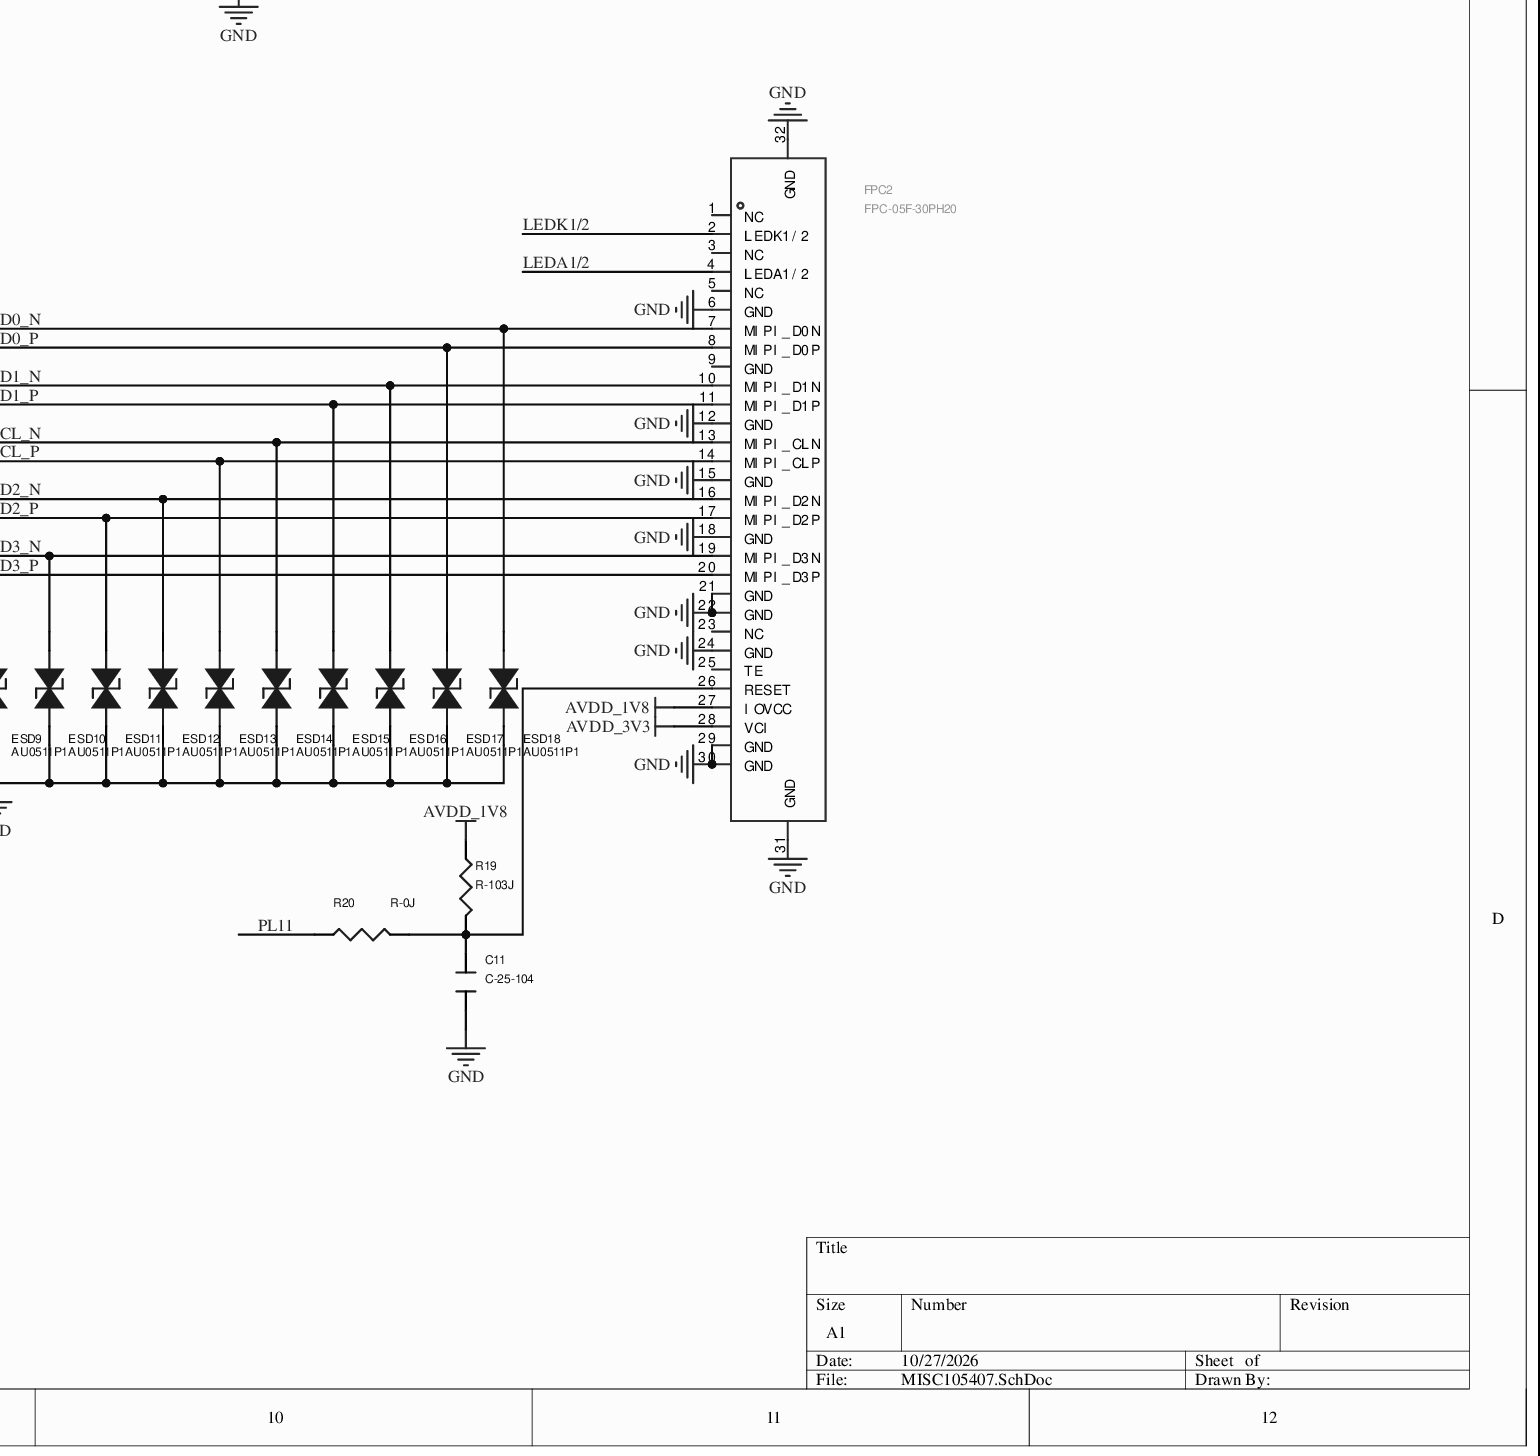
[diagram p0: MISC105407.SchDoc, bottom column 4 of 4]
# Altium project MISC105407.PrjPcb (part 3 of 3)

## Sheet MISC105407.SchDoc
size A1; SheetNumber: 1; SheetTotal: 1

### Parts
C1  C-16-225(±10%)  [C0402]
C2  C-50-104(±10%)  [C0402]
C3  C-25-104  [C0402]
C4  C-25-104  [C0402]
C5  C-25-104  [C0402]
C6  C-25-106  [C0603]
C7  C-25-104  [C0402]
C8  C-25-106  [C0603]
C9  C-25-104  [C0402]
C10  C-25-104  [C0402]
C11  C-25-104  [C0402]
C12  C-50-105  [C0402]
C13  C-25-106  [C0603]
C14  C-50-330  [C0402]
C15  C-50-104  [C0402]
C16  C-16-106(±10%)  [C0603]
C17  C-16-106(±10%)  [C0603]
C18  C-50-472(±10%)  [C0402]
C19  C-16-106(±10%)  [C0603]
C20  C-50-220(±10%)  [C0402]
C21  C-16-106(±10%)  [C0603]
C22  C-16-106(±10%)  [C0603]
C23  C-16-106(±10%)  [C0603]
C24  C-50-101  [C0402]
C25  C-50-106  [C0603]
C26  C-50-104  [C0402]
C27  C-50-330  [C0402]
D1  1N5819  [SOD323]
D2  AU0511P1  [ESD0402A]
D3  AU0511P1  [ESD0402A]
D4  1N5819  [SOD323]
D5  AU0511P1  [ESD0402A]
D6  AU0511P1  [ESD0402A]
D7  AU0511P1  [ESD0402A]
D8  AU0511P1  [ESD0402A]
D9  AU0511P1  [ESD0402A]
D10  AU0511P1  [ESD0402A]
D11  AU0511P1  [ESD0402A]
D12  AU0511P1  [ESD0402A]
D13  AU0511P1  [ESD0402A]
D14  AU0511P1  [ESD0402A]
D15  SS34F_C18199199  [SMAF_L3.5-W2.6-LS4.7-RD-1]
D16  SS34F_C18199199  [SMAF_L3.5-W2.6-LS4.7-RD-1]
D17  AU0511P1  [ESD0402A]
D18  AU0511P1  [ESD0402A]
D19  AU0511P1  [ESD0402A]
D20  AU0511P1  [ESD0402A]
D21  AU0511P1  [ESD0402A]
D22  AU0511P1  [ESD0402A]
ESD1  AU0511P1  [ESD0402A]
ESD2  AU0511P1  [ESD0402A]
ESD5  AU0511P1  [ESD0402A]
ESD6  AU0511P1  [ESD0402A]
ESD7  AU0511P1  [ESD0402A]
ESD8  AU0511P1  [ESD0402A]
ESD9  AU0511P1  [ESD0402A]
ESD10  AU0511P1  [ESD0402A]
ESD11  AU0511P1  [ESD0402A]
ESD12  AU0511P1  [ESD0402A]
ESD13  AU0511P1  [ESD0402A]
ESD14  AU0511P1  [ESD0402A]
ESD15  AU0511P1  [ESD0402A]
ESD16  AU0511P1  [ESD0402A]
ESD17  AU0511P1  [ESD0402A]
ESD18  AU0511P1  [ESD0402A]
FEL  TSB017A3126A02  [KEY-SMD_YTSB017A0312502B]
FPC1  AFC01-S08FCA-00  [FPC-SMD_P0.50-8P_FGS-XJ-H2.0]
FPC2  FPC-05F-30PH20  [FPC-SMD_30P-P0.50_XUNPU_FPC-05F-30PH20]
J1  FUET-4020  [BUZ-SMD_L4.0-W4.0-P3.50-L]
J2  TF-115-BCP9  [TF-SMD_TF-115-BCP9]
L1  10uH  [IND-SMD_L2.5-W2.0]
L2  FXL0518-2R2-M  [IND-SMD_L5.2-W5.4]
LED1  XL-3210SURUGC  [LED-SMD_4P-L3.2-W1.5_HTG-3210SURUBGC]
MIC1  GMI4015P-2C-64db  [MIC-TH_BD4.0-P1.40-D0.4-L-FD]
otg  GT-USB-9009B  [USB-C-SMD_GT-USB-9009B]
PWR  TSB017A3126A02  [KEY-SMD_YTSB017A0312502B]
Q1  S9013  [SOT23]
Q3  8050-S  [SOT-23-3]
R1  R-304J  [R0402]
R2  R-152J  [R0402]
R3  R-304F  [R0402]
R4  R-472J  [R0402]
R5  R-472J  [R0402]
R6  R-472J  [R0402]
R7  R-103J  [R0402]
R8  R-0J  [R0402]
R9  R-202J  [R0402]
R10  R-220J  [R0402]
R11  R-220J  [R0402]
R12  R-105J  [R0402]
R13  R-104J  [R0402]
R14  NC  [R0402]
R15  1M  [R0402]
R16  8R2  [R0402]
R17  8R2  [R0402]
R18  8R2  [R0402]
R19  R-103J  [R0402]
R20  R-0J  [R0402]
R21  R-103J  [R0402]
R22  R-103J  [R0402]
R23  R-102  [R0402]
R24  R-152  [R0402]
R25  R-104F  [R0402]
R26  R-202J  [R0402]
R27  R-152  [R0402]
R28  R-102  [R0402]
R29  R-103J  [R0402]
R30  R-104F  [R0402]
R31  R-202J  [R0402]
R32  R-304F  [R0402]
R33  R-332J  [R0402]
R34  R-154J  [R0402]
R35  R-622F  [R0402]
R36  R-103J  [R0402]
R37  R-103J  [R0402]
R38  R-103J  [R0402]
R39  R-5R0J  [R0402]
R40  R-103J  [R0402]
R41  R-472J  [R0402]
RST  LXTD-0204-034  [SW-SMD_LXTD-0204-034]
U1  TPS61089RNRR  [VQFN-HR_L2.5-W2.0-P0.50-TL-EP]
U2  HelperA133Core  [A133]
U3  HM5663  [SOT23-6]
U4  xc6206p182mr  [SOT23]
U8  MT9700  [SOT-23-5_L3.0-W1.7-P0.95-LS2.8-BR]
VBAT+  Header 1  [HDR-LI-1P]
VBAT-  Header 1  [HDR-LI-1P]
VIN+  Header 1  [HDR-LI-1P]
VIN-  Header 1  [HDR-LI-1P]

### Nets
AVCC: R12.1 R13.1 U2.5(AVCC)
AVDD_1V8: C10.2 FPC2.27(IOVCC) R19.1 U4.2(VOUT)
AVDD_3V3: C9.2 C13.2 D1.2(CATHODE) D6.1(ANODE) D21.1(ANODE) FPC1.3(VDD) FPC2.28(VCI) J1.1 J2.4(VDD) R4.2 R5.2 R6.2 R21.1 R22.1 R36.1 R41.2 U2.71(VCC-3V3) U4.3(VIN)
CAM_5V: C19.2 C21.2 C22.2 C23.2 R3.2 U1.6(VOUT) U8.5(VIN)
GND: C1.1 C3.2 C6.2 C7.2 C8.2 C9.1 C10.1 C11.1 C12.2 C13.1 C14.2 C16.1 C17.1 C18.2 C19.1 C20.2 C21.1 C22.1 C23.1 C27.2 D2.1(ANODE) D3.2(CATHODE) D5.2(CATHODE) D6.2(CATHODE) D7.2(CATHODE) D8.2(CATHODE) D9.2(CATHODE) D10.2(CATHODE) D11.2(CATHODE) D12.2(CATHODE) D13.2(CATHODE) D14.2(CATHODE) D17.2(CATHODE) D18.1(ANODE) D19.1(ANODE) D20.2(CATHODE) D21.2(CATHODE) D22.1(ANODE) ESD1.2(CATHODE) ESD2.2(CATHODE) ESD5.2(CATHODE) ESD6.2(CATHODE) ESD7.2(CATHODE) ESD8.2(CATHODE) ESD9.2(CATHODE) ESD10.2(CATHODE) ESD11.2(CATHODE) ESD12.2(CATHODE) ESD13.2(CATHODE) ESD14.2(CATHODE) ESD15.2(CATHODE) ESD16.2(CATHODE) ESD17.2(CATHODE) ESD18.2(CATHODE) FEL.1 FEL.3 FEL.4 FPC1.1(GND) FPC1.8(GND) FPC1.9(GND) FPC1.10(GND) FPC2.6(GND) FPC2.12(GND) FPC2.15(GND) FPC2.18(GND) FPC2.21(GND) FPC2.22(GND) FPC2.24(GND) FPC2.29(GND) FPC2.30(GND) FPC2.31(GND) FPC2.32(GND) J2.6(VSS2) J2.10(GND) J2.11(GND1) J2.12(GND2) J2.13(GND3) LED1.2(G-) LED1.4(R-) otg.25(EH) otg.26(EH) otg.27(EH) otg.28(EH) otg.A1(GND) otg.A12(GND) otg.B1(GND) otg.B12(GND) PWR.2 PWR.3 PWR.4 Q1.2(EMITTER) R7.1 R8.1 R10.2 R11.1 R14.2 R15.2 R16.2 R17.2 R18.2 R25.2 R28.2 R29.2 R33.2 R34.1 R38.2 R39.2 R40.2 RST.1 RST.3 RST.4 U1.5(GND) U2.28(GND) U2.42(GND) U2.58(GND) U2.63(GND) U2.72(GND) U2.112(GND) U2.121(GND) U3.2(GND) U4.1(GND) U8.2(GND) VBAT-.1 VIN-.1
VBAT: D20.1(ANODE) U2.107(VBAT) U2.108(VBAT) VBAT+.1
VBUS: D14.1(ANODE) otg.A4(VBUS) otg.A9(VBUS) otg.B4(VBUS) otg.B9(VBUS) U8.1(VOUT)
VCC_PS: C8.1 C16.2 C17.2 D22.2(CATHODE) L1.1 L2.1 U1.9(VIN) U2.110(PS) U3.6(IN)
VIN: D17.1(ANODE) U2.113(ACIN2) U2.114(ACIN1) VIN+.1
BEEP: R2.1 U2.83(PD10/LCD0_D14/LVDS1_D0P/SPI1_CS/PD_EINT10)
BOOST_EN: R40.1 U1.7(EN) U2.29(PH3/TWI1_SDA/CIR_OUT/RGMII0_CLKIN/RMII0_RXER/PH_EINT3)
CC1: D15.2(A) otg.A5(CC1)
CC2: D16.2(A) otg.B5(CC2)
CTP_INT: ESD6.1(ANODE) FPC1.6(INT) R6.1 U2.52(PB3/UART2_CTS/SPI2_MISO/JTAG_DI/PB_EINT3)
CTP_RST: ESD5.1(ANODE) FPC1.7(RST) R41.1 U2.51(PB2/UART2_RTS/SPI2_MOSI/JTAG_DO/PB_EINT2)
CTP_TWI1_SCK: ESD8.1(ANODE) FPC1.4(SCL) R4.1 U2.53(PB4/TWI1_SCK/I2S0_MCLK/JTAG_MS_GPU/PB_EINT4)
CTP_TWI1_SDA: ESD7.1(ANODE) FPC1.5(SDA) R5.1 U2.54(PB5/TWI1_SDA/I2S0_BCLK/JTAG_CK_GPU/PB_EINT5)
HBIAS: R9.1 U2.13(HBIAS)
HP_DET: R12.2 U2.15(HP-DET)
HPOUTFB: R8.2 U2.14(HPOUTFB)
HS_MIC: R9.2 U2.8(MIC_DET)
LCD_PWM: R15.1 U2.69(PD22/PWM1/TWI0_SCK/PD_EINT22) U3.4(~{SHDN})
LED1: R26.1 U2.47(PH13/TWI3_SDA/I2S3_MCLK/EPHY0_25/PH_EINT13)
LED2: R31.1 U2.48(PH19/CIR_IN/I2S3_DOUT3/I2S3_DIN3/LEDC/PH_EINT19)
LEDA1/2: C6.1 C7.1 D4.2(CATHODE) FPC2.4(LEDA1/2) U3.5(OVP)
LEDK1/2: FPC2.2(LEDK1/2) R14.1 R16.1 R17.1 R18.1 U3.3(FB)
LRADC: R13.2 U2.4(LRADC)
MBIAS: C12.1 R23.2 U2.18(MBIAS)
MCU_RXD: ESD2.1(ANODE) otg.A11(SSRXp2) otg.B11(SSRXp1) U2.49(PB0/UART2_TX/SPI2_CS/JTAG_MS/PB_EINT0)  [also labelled UART2_TX]
MCU_TXD: ESD1.1(ANODE) otg.A10(SSRXn2) otg.B10(SSRXn1) U2.50(PB1/UART2_RX/SPI2_CLK/JTAG_CK/PB_EINT1)  [also labelled UART2_RX]
MICIN1_N: C26.2 U2.16(MICIN1N)
MICIN1_P: C15.2 U2.17(MICIN1P)
MIPI_CL_N: ESD14.1(ANODE) FPC2.13(MIPI_CLN) U2.78(PD5/LCD0_D7/LVDS0_D2N/DSI_CKM/PD_EINT5)
MIPI_CL_P: ESD13.1(ANODE) FPC2.14(MIPI_CLP) U2.77(PD4/LCD0_D6/LVDS0_D2P/DSI_CKP/PD_EINT4)
MIPI_D0_N: ESD18.1(ANODE) FPC2.7(MIPI_D0N) U2.74(PD1/LCD0_D3/LVDS0_D0N/DSI_DM0/PD_EINT1)
MIPI_D0_P: ESD17.1(ANODE) FPC2.8(MIPI_D0P) U2.73(PD0/LCD0_D2/LVDS0_D0P/DSI_DP0/PD_EINT0)
MIPI_D1_N: ESD16.1(ANODE) FPC2.10(MIPI_D1N) U2.76(PD3/LCD0_D5/LVDS0_D1N/DSI_DM1/PD_EINT3)
MIPI_D1_P: ESD15.1(ANODE) FPC2.11(MIPI_D1P) U2.75(PD2/LCD0_D4/LVDS0_D1P/DSI_DP1/PD_EINT2)
MIPI_D2_N: ESD12.1(ANODE) FPC2.16(MIPI_D2N) U2.80(PD7/LCD0_D11/LVDS0_CKN/DSI_DM2/PD_EINT7)
MIPI_D2_P: ESD11.1(ANODE) FPC2.17(MIPI_D2P) U2.79(PD6/LCD0_D10/LVDS0_CKP/DSI_DP2/PD_EINT6)
MIPI_D3_N: ESD10.1(ANODE) FPC2.19(MIPI_D3N) U2.82(PD9/LCD0_D13/LVDS0_D3N/DSI_DM3/PD_EINT9)
MIPI_D3_P: ESD9.1(ANODE) FPC2.20(MIPI_D3P) U2.81(PD8/LCD0_D12/LVDS0_D3P/DSI_DP3/PD_EINT8)
PL11: R20.1 U2.64(PL11/S_CPU_CUR_W/S_CIR_IN/S_PL_EINT11)
SDC0_CLK: D10.1(ANODE) J2.5(CLK) U2.24(PF2/SDC0_CLK/UART0_TX/PF_EINT2)
SDC0_CMD: D11.1(ANODE) J2.3(CMD) R21.2 U2.25(PF3/SDC0_CMD/JTAG_DO/JTAG_DO_GPU/PF_EINT3)
SDC0_D0: D9.1(ANODE) J2.7(DAT0) U2.23(PF1/SDC0_D0/JTAG_DI/JTAG_DI_GPU/PF_EINT1)
SDC0_D1: D8.1(ANODE) J2.8(DAT1) U2.22(PF0/SDC0_D1/JTAG_MS/JTAG_MS_GPU/PF_EINT0)
SDC0_D2: D7.1(ANODE) J2.1(DAT2) U2.27(PF5/SDC0_D2/JTAG_CK/JTAG_CK_GPU/PF_EINT5)
SDC0_D3: D12.1(ANODE) J2.2(DAT3) U2.26(PF4/SDC0_D3/UART0_RX/PF_EINT4)
SDC0_DET: D5.1(ANODE) J2.9(CD#) R22.2 U2.21(PF6/PF_EINT6)
USB0_N: D13.1(ANODE) otg.A7(Dn1) otg.B7(Dn2) U2.105(USB0-DM)
USB0_P: D3.1(ANODE) otg.A6(Dp1) otg.B6(Dp2) U2.104(USB0-DP)
USB_HOST: R29.1 U2.30(PH10/DMIC_DATA1/SPI2_MOSI/I2S2_LRCK/MDIO0/PH_EINT10) U8.4(EN)
USB_ID: Q3.3(C) R36.2 U2.103(PH8/DMIC_CLK/SPI2_CS/I2S2_MCLK/I2S2_DIN2/PH_EINT8)
NetC1_2: C1.2 U1.2(VCC)
NetC2_1: C2.1 U1.10(BOOT)
NetC2_2: C2.2 L2.2 R1.1 U1.11(SW)
NetC3_1: C3.1 D2.2(CATHODE) PWR.1 U2.111(PWRON)
NetC4_1: C4.1 U2.9(HPOUTR)
NetC4_2: C4.2 R10.1
NetC5_1: C5.1 U2.10(HPOUTL)
NetC5_2: C5.2 R11.2
NetC11_2: C11.2 FPC2.26(RESET) R19.2 R20.2
NetC14_1: C14.1 C15.1 C24.1 R24.2 R30.1
NetC18_1: C18.1 R35.1 U1.4(COMP)
NetC20_1: C20.1 R35.2
NetC24_2: C24.2 C26.1 C27.1 R27.2 R32.1
NetC25_1: C25.1 R23.1 R24.1
NetC25_2: C25.2 R27.1 R28.1
NetD1_1: D1.1(ANODE) J1.2 Q1.3(COLLECTOR)
NetD4_1: D4.1(ANODE) L1.2 U3.1(SW)
NetD15_1: D15.1(K) D16.1(K) R37.2
NetD18_2: D18.2(CATHODE) MIC1.2(-) R32.2
NetD19_2: D19.2(CATHODE) MIC1.1(+) R30.2
NetFEL_2: FEL.2 U2.2(FEL)
NetLED1_1: LED1.1(G+) R26.2
NetLED1_3: LED1.3(R+) R31.2
NetQ1_1: Q1.1(BASE) R2.2
NetQ3_1: Q3.1(B) R37.1 R38.1
NetQ3_2: Q3.2(E) R39.1
NetR1_2: R1.2 U1.1(FSW)
NetR3_1: R3.1 R25.1 U1.3(FB)
NetR7_2: R7.2 U2.109(TS)
NetR33_1: R33.1 U8.3(SET)
NetR34_2: R34.2 U1.8(ILIM)
NetRST_2: RST.2 U2.3(RESET)

Not connected (* = marked no-connect by the designer): FPC1 2(NC); FPC2 1(NC) 3(NC) 5(NC) 9(GND) 23(NC) 25(TE); otg A2(SSTXp1) A3(SSTXn1) A8(SUB1) B2(SSTXp2) B3(SSTXn2) B8(SUB2); U2 1(IOVDD-CSI) 6(LINEOUTLN) 7(LINEOUTLP) 11(MICIN2N) 12(MICIN2P) 19(PB7/SPDIF_IN/I2S0_DOUT0/I2S0_DIN1/PB_EINT7) 20(PB8/SPDIF_OUT/I2S0_DIN0/I2S0_DOUT1/PB_EINT8) 31(PH9/DMIC_DATA0/SPI2_CLK/I2S2_BCLK/MDC0/PH_EINT9) 32(PH11/DMIC_DATA2/SPI2_MISO/I2S2_DOUT0/I2S2_DIN1/PH_EINT11) 33(PH7/UART3_CTS/SPI1_MISO/SPDIF_OUT/RGMII0_TXCTL/RMII0_TXEN/PH_EINT7) 34(PH17/I2S3_DOUT1/I2S3_DIN0/RGMII0_TXD3/RMII0_NULL/PH_EINT17) 35(PH18/CIR_OUT/I2S3_DOUT2/I2S3_DIN2/RGMII0_TXD2/RMII0_NULL/PH_EINT18) 36(PH4/UART3_TX/SPI1_CS/CPU_CUR_W/RGMII0_TXD1/RMII0_TXD1/PH_EINT4) 37(PH5/UART3_RX/SPI1_CLK/LEDC/RGMII0_TXD0/RMII0_TXD0/PH_EINT5) 38(PH6/UART3_RTS/SPI1_MOSI/SPDIF_IN/RGMII0_TXCK/RMII0_TXCK/PH_EINT6) 39(PH16/I2S3_DOUT0/I2S3_DIN1/RGMII0_RXCK/RMII0_NULL/PH_EINT16) 40(PH14/I2S3_BCLK/RGMII0_RXD3/RMII0_NULL/PH_EINT14) 41(PH15/I2S3_LRCK/RGMII0_RXD2/RMII0_NULL/PH_EINT15) 43(PH0/TWI0_SCK/RGMII0_RXD1/RMII0_RXD1/PH_EINT0) 44(PH1/TWI0_SDA/RGMII0_RXD0/RMII0_RXD0/PH_EINT1) 45(PH2/TWI1_SCK/CPU_CUR_W/RGMII0_RXCTL/RMII0_CRS_DV/PH_EINT2) 46(PH12/DMIC_DATA3/TWI3_SCK/I2S2_DIN0/I2S2_DOUT1/PH_EINT12) 55(PB6/I2S0_LRCK/JTAG_DO_GPU/PB_EINT6) 56(PB9/UART0_TX/TWI0_SCK/JTAG_DI_GPU/PB_EINT9) 57(PB10/UART0_RX/TWI0_SDA/PWM1/PB_EINT10) 59(PG9/UART1_CTS/I2S1_MCLK/PG_EINT9) 60(PG8/UART1_RTS/PG_EINT8) 61(PG7/UART1_RX/PG_EINT7) 62(PG6/UART1_TX/PG_EINT6) 65(PL10/S_PWM/S_PL_EINT10) 66(PL9/S_TWI1_SDA/S_PL_EINT9) 67(PL8/S_TWI1_SCK/S_PL_EINT8) 68(PL7/S_JTAG_DI/S_PL_EINT7) 70(CHGLED) 84(PD11/LCD0_D15/LVDS1_D0N/SPI1_CLK/PD_EINT11) 85(PD12/LCD0_D18/LVDS1_D1P/SPI1_MOSI/PD_EINT12) 86(PD13/LCD0_D19/LVDS1_D1N/SPI1_MISO/PD_EINT13) 87(PD14/LCD0_D20/LVDS1_D2P/UART3_TX/PD_EINT14) 88(PD15/LCD0_D21/LVDS1_D2N/UART3_RX/PD_EINT15) 89(PD16/LCD0_D22/LVDS1_CKP/PLL_TEST_CKP/UART3_RTS/PD_EINT16) 90(PD17/LCD0_D23/LVDS1_CKN/PLL_TEST_CKN/UART3_CTS/PD_EINT17) 91(PD18/LCD0_CLK/LVDS1_D3P/UART4_TX/PD_EINT18) 92(PD19/LCD0_DE/LVDS1_D3N/UART4_RX/PD_EINT19) 93(PD20/LCD0_HSYNC_/PWM2/UART4_RTS/PD_EINT20) 94(PD21/LCD0_VSYNC/PWM3/UART4_CTS/PD_EINT21) 95(PD23/PWM0/TWI0_SDA/PD_EINT23) 96(PC12/NAND_DQS/SPI0_CLK/PC_EINT12) 97(PC7/NAND_RB1/SPI0_CS1/PC_EINT7) 98(PC4/NAND_CE0/SPI0_MISO/PC_EINT4) 99(PC3/NAND_CE1/SPI0_CS0/PC_EINT3) 100(PC2/NAND_CLE/SPI0_MOSI/PC_EINT2) 101(USB1-DP) 102(USB1-DM) 106(VBUS) 115(PE9/BIST_RESULT3/I2S2_DIN0/PE_EINT9) 116(PE8/BIST_RESULT2/I2S2_DOUT0/PE_EINT8) 117(PE7/CSI_SM_VS/BIST_RESULT1/I2S2_LRCK/TCON_TRIG/PE_EINT7) 118(PE6/BIST_RESULT0/I2S2_BCLK/PE_EINT6) 119(PE4/TWI3_SDA/PE_EINT4) 120(PE3/TWI3_SCK/PE_EINT3) 122(MCSIA_D3N) 123(MCSIA_D3P) 124(MCSIA_D2N) 125(MCSIA_D2P) 126(MCSIA_D1N) 127(MCSIA_D1P) 128(MCSIA_D0N) 129(MCSIA_D0P) 130(MCSIA_CLKN) 131(MCSIA_CLKP) 132(MCSIB_D1N) 133(MCSIB_D1P) 134(MCSIB_D0N) 135(MCSIB_D0P) 136(MCSIB_CLKN) 137(MCSIB_CLKP) 138(PE5/MIPI_MCLK1/PLL_LOCK_DBG/I2S2_MCLK/LEDC/PE_EINT5) 139(PE0/MIPI_MCLK0/PE_EINT0) 140(PE1/TWI2_SCK/PE_EINT1) 141(PE2/TWI2_SDA/PE_EINT2) 142(AFVCC-CSI) 143(DVDD-CSI) 144(AVDD-CSI)

### Layout directives
differential pair: MICIN1_N, MICIN1_P, MIPI_CL_N, MIPI_CL_P, MIPI_D0_N, MIPI_D0_P, MIPI_D1_N, MIPI_D1_P, MIPI_D2_N, MIPI_D2_P, MIPI_D3_N, MIPI_D3_P, USB0_N, USB0_P

### Notes on the sheet
- Component
- Diferential
- single-ended
- R3
- R1 R2 C1
  C3 D1
- USE
- NC
- (near MIC1) -
- (near MIC1) +
- (near C24) C1
- C3
- C2
- 1.5K
- 33pF
- 1K
- 0R
- (near D18) D1
- (near C27) C2
- R1
- R2
- Close to MIC
- Close to AP
- (near R8) Note:
  必须保留电路，
  HPOUTFB 接个0R电阻到GND，
  HS-MIC与HBIAS之间用一个2K电阻相连接。
  HP-DET与AVCC之间接个1M上拉电阻
  LRADC与AVCC之间接个100K电阻
- (near U2) 注：
  TS，电池温度检测脚。
  无此功能时接个10K电阻到地。
- 注意
  HPOUTL/HPOUTR引脚，
  用不用都必须接这个电路
- (near U2) 3.3V  PB PH PF
- 1.8V  PL PC PG
- Core board supply current must be above 1.5A.
- SDIO2.0

### Library data of the parts
C1-C8 C18 C20 = C-XX-XXX: Chip capacitor; Text Field1: 20; D/S: S; Text Field2: 20
C9 C10 = CAP NP_0: Status: Taiwan
C11 C13 = CAPACITOR_0: PAGE: 2
C12 C15 C24 C26 = C-C0402-X5R_0: Parameter: C0402-X5R
C14 C27 = C-C0402-COG_0: Parameter: C0402-COG
C16 C17 C19 C21-C23 = C-XX-XXX: Chip capacitor; Text Field1: 20; D/S: S; PN: GRM1555C1H270J; Text Field2: 20
C25 = C-C0603-X5R_1: Parameter: C0603-X5R
D1 D4 = BAS21/SOT_1
D2 D3 D5-D14 D17 D20-D22 ESD1 ESD2 ESD5-ESD18 = 1_1.5KE100A: 1ST PART DESCRIPTION: WILL ESD9B5V Bidirection ESD Protection
D18 D19 = ESD9B5VL: ID: DE-E0001; Parameter: ESD0402; options: 4890-1
FPC1 = FPC-05F-8PH20: Manufacturer: JS(钜硕电子); Add into BOM: yes; Locking Feature: Flip-lock; Number of Contacts: 8P; Pitch: 0.5mm; FFC, FCB Thickness: 0.3mm; Symbol: AFC01-S08FCA-00; Device: AFC01-S08FCA-00; LCSC Part Name: 间距:0.5mm P数:8P 翻盖式 下接; Supplier Part: C262657; Manufacturer Part: AFC01-S08FCA-00; Supplier Footprint: SMD,P=0.5mm,卧贴; JLCPCB Part Class: Extended Part; Datasheet: https://item.szlcsc.com/datasheet/AFC01-S08FCA-00/253916.html; Supplier: LCSC; Convert to PCB: yes; Contact Type: Bottom entry; Mounting Type: Horizontal SMT; Height Above Board: 2mm
FPC2 = FPC-05F-30PH20: Manufacturer: XUNPU(讯普); Add into BOM: yes; Locking Feature: Flip-lock; Number of Contacts: 30P; Pitch: 0.5mm; FFC, FCB Thickness: 0.3mm; Rated Voltage (Max): 50V; Current Rating (Max): 500mA; Symbol: FPC-05F-30PH20; Device: FPC-05F-30PH20; LCSC Part Name: 翻盖式 卧贴 P数:30P 间距:0.5mm; Supplier Part: C2856808; Manufacturer Part: FPC-05F-30PH20; Supplier Footprint: SMD,P=0.5mm,卧贴; JLCPCB Part Class: Extended Part; Datasheet: https://item.szlcsc.com/datasheet/FPC-05F-30PH20/3056906.html; Supplier: LCSC; Convert to PCB: yes; Contact Type: Horizontal SMT; Mounting Type: Bottom entry; Height Above Board: 2mm; Contact Material: Phosphor bronze; Contact Plating: Tin; Operating Temperature: -25℃~+85℃
J1 = CON2_0
J2 = SDMMC SLOT_0
L1 = INDUCTOR
L2 = L: Low-power chip inductor; BOM名称: Low-power chip inductor
MIC1 = Micphone_0: mypage: 13
otg = TYPE-C-31-M-01: Manufacturer: 韩国韩荣; Add into BOM: yes; Connector Type: Type-C; Gender: Female; Number of Ports: 1; Number of Contacts: 24P; Symbol: TYPE-C-31-M-01; Device: TYPE-C-31-M-01; LCSC Part Name: Type-C 母 沉板; Supplier Part: C129016; Manufacturer Part: TYPE-C-31-M-01; Supplier Footprint: SMD; JLCPCB Part Class: Extended Part; Datasheet: https://atta.szlcsc.com/upload/public/pdf/source/20210810/7B555BB1ED5795CFEF9B6A492F7A3536.pdf; Supplier: LCSC; Convert to PCB: yes; Standard: -; Mounting Style: Board-sunk; Current Rating - Power (Max): -; Operating Temperature Range: -55℃~+85℃
Q1 = 2N3904_0
Q3 = 8050-S: NPN transistor; Manufacturer: Generic Components; Class: Discrete; SubClass: BJT - Low Power; D/S: S; Published: 08/06/2000; Publisher: Altium Hobart Technology Centre
R1 R3 R25 R30 R32 R34 R35 = R-XXXJ: Chip resistor
R2 = R_Dup2
R4-R6 R14-R18 R20 R41 = R
R7-R13 R26 R29 R31 R33 R36-R40 = R-XXXJ: Chip resistor; D/S: S
R19 R21 R22 = R_Dup7
R23 R24 R27 R28 = R-R0402-5%_Dup1
RST = TSB017A3126A02: Symbol: TSB017A3126A02
U1 = TPS61089RNRR: Manufacturer: TI(德州仪器); Add into BOM: yes; Function: Boost; Output Type: Adjustable; Input Voltage: 2.7V~12V; Output Voltage: 4.5V~12.6V; Output Current: 7A; Switching Frequency: 2.2MHz; Number of Outputs: 1; Switch tube (built-in/external): Built-in; Symbol: TPS61089RNRR; Device: TPS61089RNRR; LCSC Part Name: 12.6V,7A全集成同步升压转换器; Supplier Part: C165129; Manufacturer Part: TPS61089RNRR; Supplier Footprint: VQFN-11-HR-EP(2x2.5); JLCPCB Part Class: Extended Part; Datasheet: https://www.ti.com/cn/lit/gpn/tps61089; Supplier: LCSC; Convert to PCB: yes; Operating Temperature: -40℃~+125℃@(TJ); Synchronous Rectification: Yes; Topology: Boost
U2 = SOC2416_8: Manufacturer: MPS; Voltage: 2000V; Mfg #1: KEMET; Toler.: 10%; Watts: 0.1W; Part Type: 2416 core board
U3 = PT4110_0
U4 = SGM2028_0: ID: U-IC0031; Parameter: SOT23-5,input 2.5~5.5V,current=0.5A
VBAT+ VBAT- VIN+ VIN- = Header 1: 1P
D15 D16 = SS34F_C18199199: Symbol: SS34F_C18199199
FEL PWR = TSB017A3126A02: Symbol: TSB017A3126A02
LED1 = XL-3210SURUGC: Symbol: XL-3210SURUGC
U8 = MT9700: Symbol: MT9700